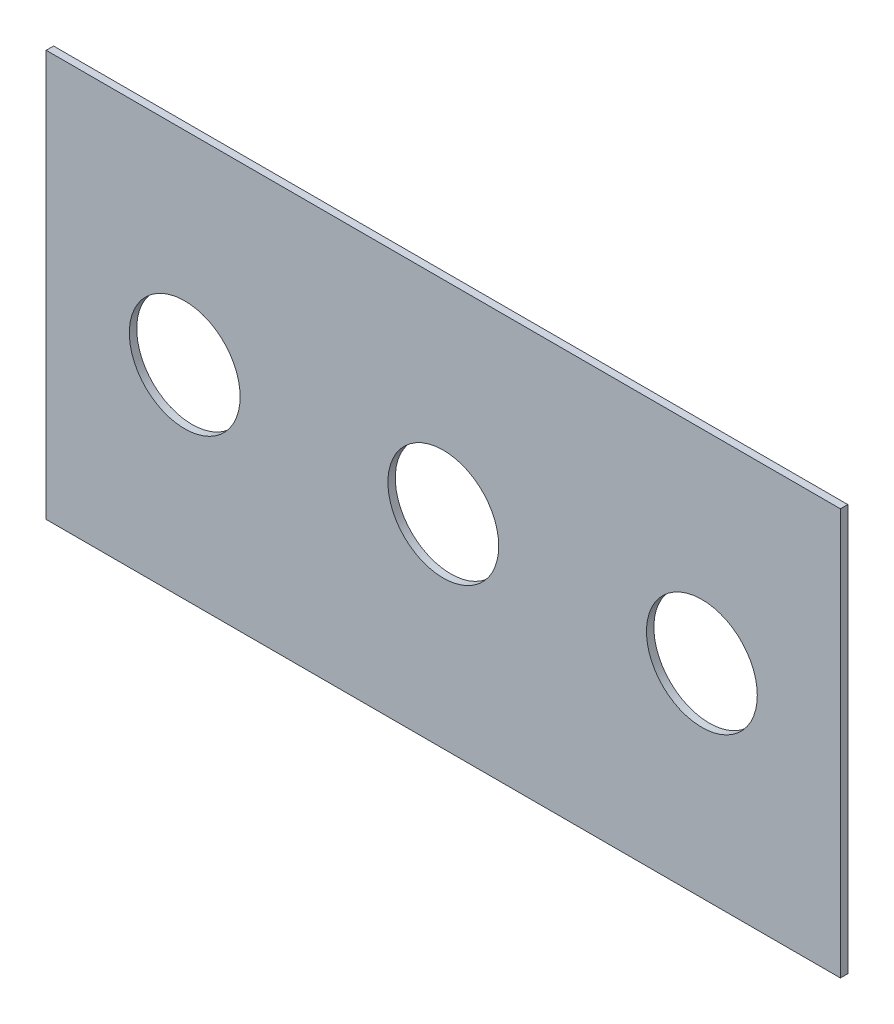
from build123d import *

# Parameters (mm, degrees)
SKETCH_1_W          = 43
SKETCH_1_H          = 22
EXTRUDE_1_DEPTH     = 0.4
SKETCH_2_R          = 3
CUT_EXTRUDE_1_DEPTH = 0.4


with BuildPart() as part:
    # 草图1 → 凸台-拉伸1 (new body)
    with BuildSketch(Plane.XY):
        Rectangle(SKETCH_1_W, SKETCH_1_H)
    extrude(amount=EXTRUDE_1_DEPTH)

    # 草图2 → 切除-拉伸1 (cut)
    with BuildSketch(Plane.XY.offset(0.4)):
        Circle(SKETCH_2_R)
        with Locations((-14, 0)):
            Circle(SKETCH_2_R)
        with Locations((14, 0)):
            Circle(SKETCH_2_R)
    extrude(amount=-CUT_EXTRUDE_1_DEPTH, mode=Mode.SUBTRACT)


solid = part.part
